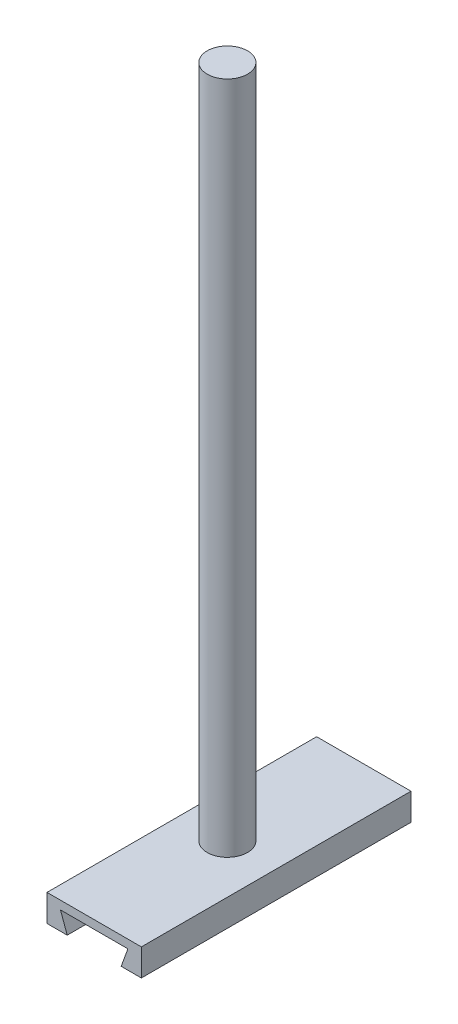
SolidWorks part; units mm, degrees
material "普通碳钢"
ref_plane "Front Plane" through (0, 0, 0) normal (0, 0, 1) x (1, 0, 0)
ref_plane "Top Plane" through (0, 0, 0) normal (0, 1, 0) x (1, 0, 0)
ref_plane "Right Plane" through (0, 0, 0) normal (1, 0, 0) x (0, 0, -1)
sketch "Sketch1" plane through (0, 0, 0) normal (0, 0, 1) x (1, 0, 0)
  line L0 (-30.2622, 19.2191) -> (39.7378, 19.2191)
  line L1 (39.7378, 19.2191) -> (39.7378, -0.7809)
  line L2 (39.7378, -0.7809) -> (24.7378, -0.7809)
  line L3 (24.7378, -0.7809) -> (29.7378, 12.9565)
  line L4 (29.7378, 12.9565) -> (-20.2622, 12.9565)
  line L5 (-20.2622, 12.9565) -> (-15.2622, -0.7809)
  line L6 (-15.2622, -0.7809) -> (-30.2622, -0.7809)
  line L7 (-30.2622, -0.7809) -> (-30.2622, 19.2191)
  dimension "D1" = 20
  dimension "D2" = 70
  dimension "D3" = 50
  dimension "D4" = 70
  dimension "D5" = 15
  dimension "D6" = 15
  dimension "D7" = 70
extrude "Boss-Extrude1" add sketch "Sketch1" along normal blind 200
sketch "Sketch2" plane through (0, 19.2191, 0) normal (0, 1, 0) x (1, 0, 0)
  circle A0 centre (3.5244, -100) radius 15
  dimension "D1" = 30
extrude "Boss-Extrude2" add sketch "Sketch2" along normal blind 500
